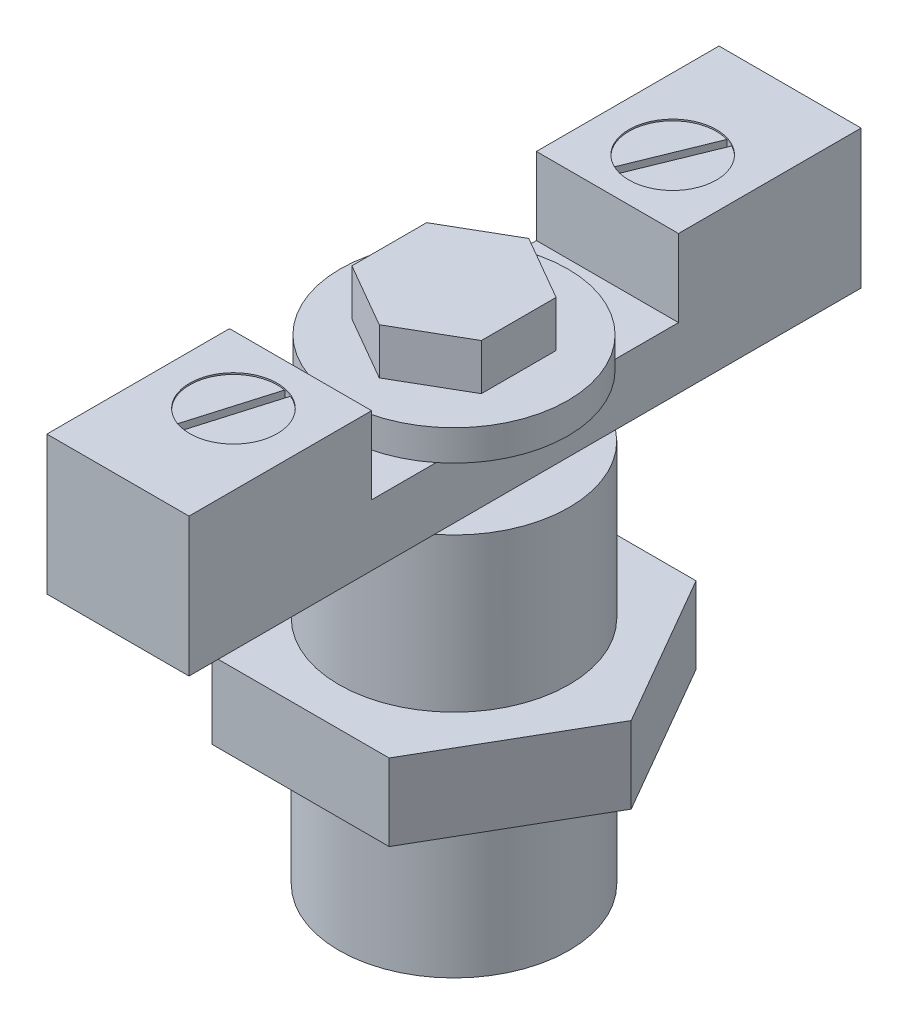
from build123d import *

# Parameters (mm, degrees)
BOSS_EXTRUDE1_DEPTH = 5
SKETCH2_R           = 7.5
BOSS_EXTRUDE2_DEPTH = 10
BOSS_EXTRUDE7_START = 10
SKETCH9_R           = 7.5
BOSS_EXTRUDE7_DEPTH = 10
SKETCH3_W           = 9.261773254
SKETCH3_H           = 43.8
BOSS_EXTRUDE3_DEPTH = 4
SKETCH4_W           = 9.261773254
SKETCH4_H           = 11.9
BOSS_EXTRUDE4_DEPTH = 5.03
SKETCH5_R           = 7.423962758
BOSS_EXTRUDE5_DEPTH = 2
BOSS_EXTRUDE6_DEPTH = 3
SKETCH7_R           = 2.850666807
CUT_EXTRUDE1_DEPTH  = 0.1
CUT_EXTRUDE2_DEPTH  = 1


with BuildPart() as part:
    # Sketch1 → Boss-Extrude1 (new body)
    with BuildSketch(Plane(origin=(0, 0, 0), x_dir=(1, 0, 0), z_dir=(0, 1, 0))):
        Polygon((5.773502692, 10), (-5.773502692, 10), (-11.547005384, 0), (-5.773502692, -10), (5.773502692, -10), (11.547005384, 0), align=None)
    extrude(amount=BOSS_EXTRUDE1_DEPTH)

    # Sketch2 → Boss-Extrude2 (add)
    with BuildSketch(Plane.XZ):
        with Locations(Location((0, 0, 0), (0, 0, 270))):
            Circle(SKETCH2_R)
    extrude(amount=BOSS_EXTRUDE2_DEPTH)

    # Sketch9 → Boss-Extrude7 (add)
    with BuildSketch(Plane(origin=(0, 5, 0), x_dir=(1, 0, 0), z_dir=(0, 1, 0)).offset(BOSS_EXTRUDE7_START)):
        with Locations(Location((0, 0, 0), (0, 0, 90))):
            Circle(SKETCH9_R)
    extrude(amount=-BOSS_EXTRUDE7_DEPTH)

    # Sketch3 → Boss-Extrude3 (add)
    with BuildSketch(Plane(origin=(0, 15, 0), x_dir=(1, 0, 0), z_dir=(0, 1, 0))):
        Rectangle(SKETCH3_W, SKETCH3_H)
    extrude(amount=BOSS_EXTRUDE3_DEPTH)

    # Sketch4 → Boss-Extrude4 (add)
    with BuildSketch(Plane(origin=(0, 19, 0), x_dir=(1, 0, 0), z_dir=(0, 1, 0))):
        with Locations((0, 15.95)):
            Rectangle(SKETCH4_W, SKETCH4_H)
        with Locations((0, -15.95)):
            Rectangle(SKETCH4_W, SKETCH4_H)
    extrude(amount=BOSS_EXTRUDE4_DEPTH)

    # Sketch5 → Boss-Extrude5 (add)
    with BuildSketch(Plane(origin=(0, 19, 0), x_dir=(1, 0, 0), z_dir=(0, 1, 0))):
        with Locations(Location((0, 0, 0), (0, 0, 51.407625877))):
            Circle(SKETCH5_R)
    extrude(amount=BOSS_EXTRUDE5_DEPTH)

    # Sketch6 → Boss-Extrude6 (add)
    with BuildSketch(Plane(origin=(0, 21, 0), x_dir=(1, 0, 0), z_dir=(0, 1, 0))):
        Polygon((0, 4.871086868), (-4.218484972, 2.435543434), (-4.218484972, -2.435543434), (0, -4.871086868), (4.218484972, -2.435543434), (4.218484972, 2.435543434), align=None)
    extrude(amount=BOSS_EXTRUDE6_DEPTH)

    # Sketch7 → Cut-Extrude1 (cut)
    with BuildSketch(Plane(origin=(0, 24.03, 0), x_dir=(1, 0, 0), z_dir=(0, 1, 0))):
        with Locations(Location((0, 14.250511049, 0), (0, 0, 270))):
            Circle(SKETCH7_R)
        with Locations(Location((0, -14.372767949, 0), (0, 0, 270))):
            Circle(SKETCH7_R)
    extrude(amount=-CUT_EXTRUDE1_DEPTH, mode=Mode.SUBTRACT)

    # Sketch8 → Cut-Extrude2 (cut)
    with BuildSketch(Plane(origin=(0, 23.93, 0), x_dir=(1, 0, 0), z_dir=(0, 1, 0))):
        Polygon((-1.343066927, 11.719300444), (0.804329856, 17.000767289), (1.330666503, 16.786763555), (-0.81673028, 11.505296711), align=None)
        Polygon((-1.076876675, -17.027451515), (0.531783037, -11.557769723), (1.076876675, -11.718084383), (-0.531783037, -17.187766175), align=None)
    extrude(amount=-CUT_EXTRUDE2_DEPTH, mode=Mode.SUBTRACT)


solid = part.part
